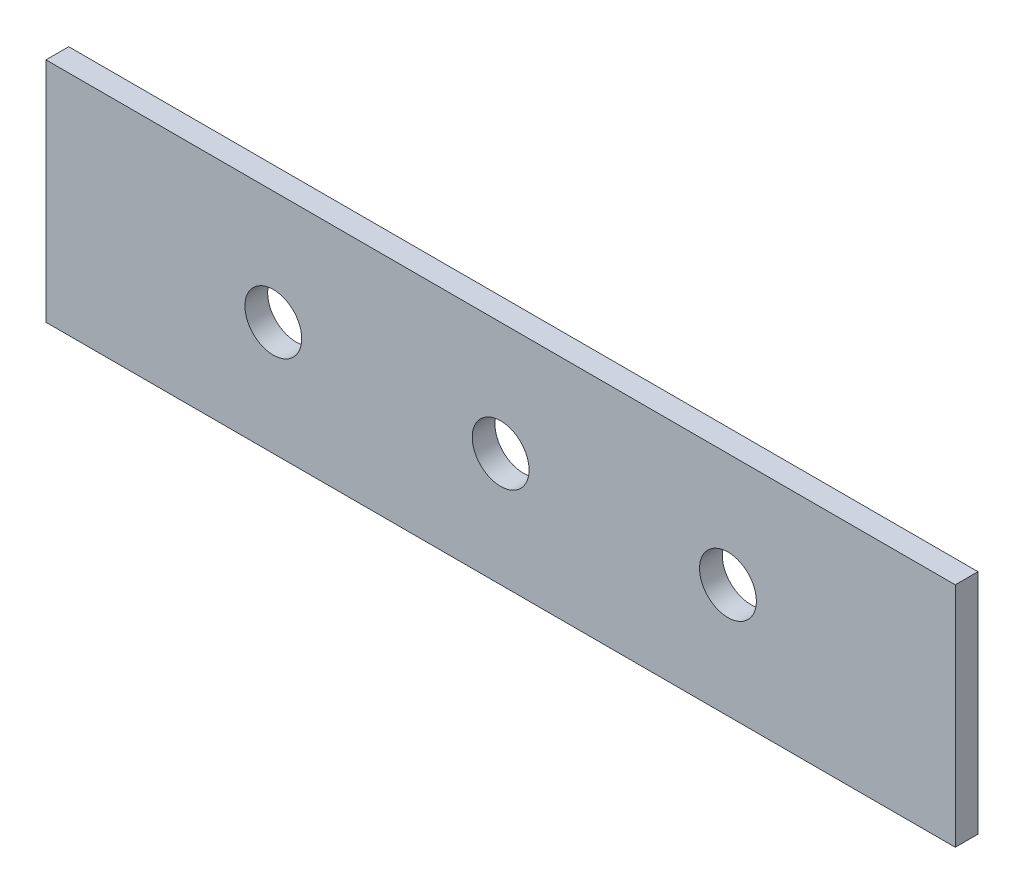
from build123d import *

# Parameters (mm, degrees)
EXTRUDE_1_DEPTH     = 8
SKETCH_2_R          = 10
CUT_EXTRUDE_1_DEPTH = 24


with BuildPart() as part:
    # 草图1 → 凸台-拉伸1 (new body)
    with BuildSketch(Plane.XY):
        Polygon((0, 0), (0, 80), (310, 80), (320, 80), (320, 0), align=None)
    extrude(amount=EXTRUDE_1_DEPTH)

    # 草图2 → 切除-拉伸1 (cut)
    with BuildSketch(Plane.XY.offset(8)):
        with Locations((80, 40)):
            Circle(SKETCH_2_R)
        with Locations((160, 40)):
            Circle(SKETCH_2_R)
        with Locations((240, 40)):
            Circle(SKETCH_2_R)
    extrude(amount=-CUT_EXTRUDE_1_DEPTH, mode=Mode.SUBTRACT)


solid = part.part
